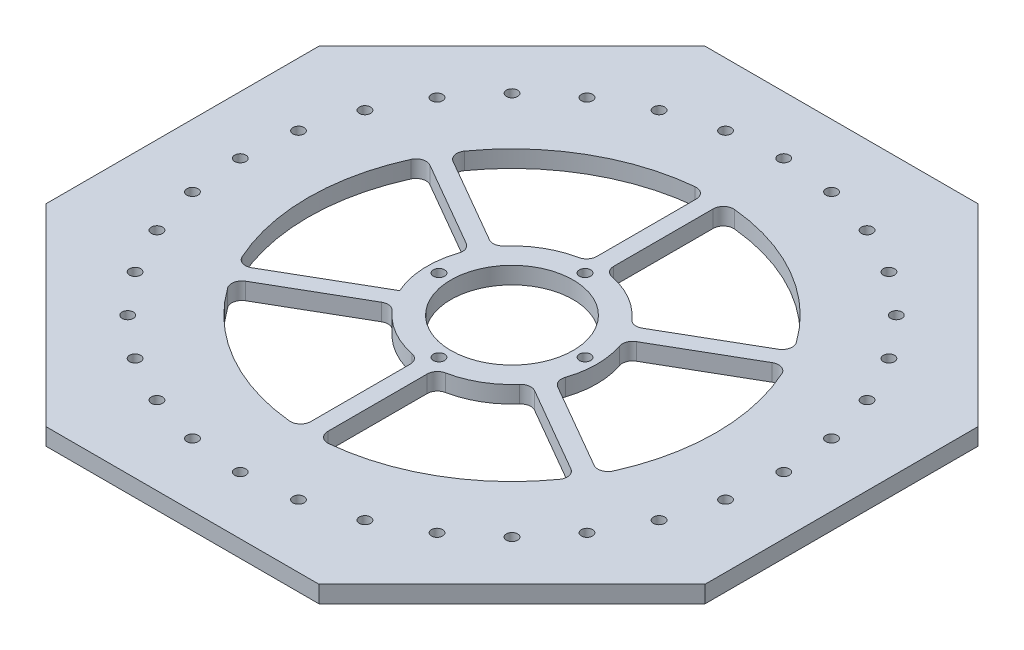
from build123d import *

# Parameters (mm, degrees)
SKETCH_1_R               = 25
SKETCH_1_R_2             = 18
EXTRUDE_1_DEPTH          = 2.5
SKETCH_1_R_3             = 60
EXTRUDE_1_2_DEPTH        = 2.5
SKETCH_8_W               = 5
SKETCH_8_H               = 39.844025058
EXTRUDE_2_DEPTH          = 5
PATTERN_CIRCULAR_3_COUNT = 6
EXTRUDE_START            = 12
SKETCH_9_R               = 25
SKETCH_9_R_2             = 18
EXTRUDE_3_DEPTH          = 12
SKETCH_11_R              = 1.65
CUT_EXTRUDE_3_DEPTH      = 8
PATTERN_CIRCULAR_5_COUNT = 32
SKETCH_12_R              = 2.2
CUT_EXTRUDE_4_DEPTH      = 45
CUT_EXTRUDE_START        = -24
SKETCH_13_R              = 4
CUT_EXTRUDE_5_DEPTH      = 45
PATTERN_CIRCULAR_6_COUNT = 4
SKETCH_14_R              = 25
CUT_EXTRUDE_6_DEPTH      = 12
FILLET_1_R               = 3
SKETCH_15_R              = 1.65
CUT_EXTRUDE_7_DEPTH      = 10
PATTERN_CIRCULAR_7_COUNT = 4


with BuildPart() as part:
    # 草图1 → 凸台-拉伸1 (new, symmetric)
    with BuildSketch(Plane(origin=(0, 0, 0), x_dir=(1, 0, 0), z_dir=(0, 1, 0))):
        with Locations(Location((0, 0, 0), (0, 0, 270))):
            Circle(SKETCH_1_R)
        with Locations(Location((0, 0, 0), (0, 0, 270))):
            Circle(SKETCH_1_R_2, mode=Mode.SUBTRACT)
    extrude(amount=EXTRUDE_1_DEPTH, both=True)



with BuildPart() as body_2:
    # 草图1 → Extrude 1 2 (new, symmetric)
    with BuildSketch(Plane(origin=(0, 0, 0), x_dir=(1, 0, 0), z_dir=(0, 1, 0))):
        Polygon((97.007350914, 40.181760398), (40.181760398, 97.007350914), (-40.181760398, 97.007350914), (-97.007350914, 40.181760398), (-97.007350914, -40.181760398), (-40.181760398, -97.007350914), (40.181760398, -97.007350914), (97.007350914, -40.181760398), align=None)
        with Locations(Location((0, 0, 0), (0, 0, 270))):
            Circle(SKETCH_1_R_3, mode=Mode.SUBTRACT)
    extrude(amount=EXTRUDE_1_2_DEPTH, both=True)


with BuildPart() as part_1:
    add(part.part)

    add(body_2.part)  # 凸台-拉伸2 merges body 2
    # 草图8 → 凸台-拉伸2 (add)
    with BuildSketch(Plane(origin=(0, 2.5, 0), x_dir=(1, 0, 0), z_dir=(0, 1, 0))):
        with Locations((0, 44.796698457)):
            Rectangle(SKETCH_8_W, SKETCH_8_H)
    extrude_2 = extrude(amount=-EXTRUDE_2_DEPTH)

    # 阵列(圆周)3: 凸台-拉伸2 ×6 about axis
    pattern_circular_3_axis = Axis((0, 0, 0), (0, 1, 0))
    for i in range(1, PATTERN_CIRCULAR_3_COUNT):
        add(extrude_2.rotate(pattern_circular_3_axis, i * 360 / PATTERN_CIRCULAR_3_COUNT))

    # 草图9 → 凸台-拉伸3 (add)
    with BuildSketch(Plane(origin=(0, 2.5, 0), x_dir=(1, 0, 0), z_dir=(0, 1, 0)).offset(EXTRUDE_START)):
        with Locations(Location((0, 0, 0), (0, 0, 84.260829523))):
            Circle(SKETCH_9_R)
        with Locations(Location((0, 0, 0), (0, 0, 270))):
            Circle(SKETCH_9_R_2, mode=Mode.SUBTRACT)
    extrude(amount=-EXTRUDE_3_DEPTH)

    # 草图11 → 切除-拉伸3 (cut)
    with BuildSketch(Plane(origin=(0, 2.5, 0), x_dir=(1, 0, 0), z_dir=(0, 1, 0))):
        with Locations(Location((0, 80, 0), (0, 0, 270))):
            Circle(SKETCH_11_R)
    cut_extrude_3 = extrude(amount=-CUT_EXTRUDE_3_DEPTH, mode=Mode.SUBTRACT)

    # 阵列(圆周)5: 切除-拉伸3 ×32 about axis
    pattern_circular_5_axis = Axis((0, 0, 0), (0, 1, 0))
    for i in range(1, PATTERN_CIRCULAR_5_COUNT):
        add(cut_extrude_3.rotate(pattern_circular_5_axis, i * 360 / PATTERN_CIRCULAR_5_COUNT), mode=Mode.SUBTRACT)

    # 草图12 → 切除-拉伸4 (cut)
    with BuildSketch(Plane.XY):
        with Locations(Location((0, 9.5, 0), (0, 0, 90))):
            Circle(SKETCH_12_R)
    cut_extrude_4 = extrude(amount=-CUT_EXTRUDE_4_DEPTH, mode=Mode.SUBTRACT)

    # 草图13 → 切除-拉伸5 (cut)
    with BuildSketch(Plane.XY.offset(CUT_EXTRUDE_START)):
        with Locations((0, 9.5)):
            Circle(SKETCH_13_R)
    cut_extrude_5 = extrude(amount=-CUT_EXTRUDE_5_DEPTH, mode=Mode.SUBTRACT)

    # 阵列(圆周)6: 切除-拉伸4, 切除-拉伸5 ×4 about axis
    pattern_circular_6_axis = Axis((0, 0, 0), (0, 1, 0))
    add([cut_extrude_4.rotate(pattern_circular_6_axis, i * 360 / PATTERN_CIRCULAR_6_COUNT) for i in range(1, PATTERN_CIRCULAR_6_COUNT)], mode=Mode.SUBTRACT)
    add([cut_extrude_5.rotate(pattern_circular_6_axis, i * 360 / PATTERN_CIRCULAR_6_COUNT) for i in range(1, PATTERN_CIRCULAR_6_COUNT)], mode=Mode.SUBTRACT)

    # 草图14 → 切除-拉伸6 (cut)
    with BuildSketch(Plane(origin=(0, 14.5, 0), x_dir=(1, 0, 0), z_dir=(0, 1, 0))):
        Circle(SKETCH_14_R)
    extrude(amount=-CUT_EXTRUDE_6_DEPTH, mode=Mode.SUBTRACT)

    # 圆角1
    fillet_1_edges = [part_1.edges().sort_by_distance(p)[0] for p in [
        (2.5, 0, 59.947894041),
        (2.5, 0, 24.874685928),
        (-2.5, 0, 59.947894041),
        (-2.5, 0, 24.874685928),
        (-50.666399143, 0, 32.13901053),
        (-20.292109925, 0, 14.602406473),
        (-53.166399143, 0, 27.808883511),
        (-53.166399143, 0, -27.808883511),
        (-22.792109925, 0, -10.272279454),
        (-50.666399143, 0, -32.13901053),
        (-20.292109925, 0, -14.602406473),
        (-2.5, 0, -59.947894041),
        (-2.5, 0, -24.874685928),
        (2.5, 0, -59.947894041),
        (2.5, 0, -24.874685928),
        (50.666399143, 0, -32.13901053),
        (20.292109925, 0, -14.602406473),
        (53.166399143, 0, -27.808883511),
        (22.792109925, 0, -10.272279454),
        (53.166399143, 0, 27.808883511),
        (22.792109925, 0, 10.272279454),
        (50.666399143, 0, 32.13901053),
        (20.292109925, 0, 14.602406473),
    ]]
    fillet(fillet_1_edges, radius=FILLET_1_R)

    # 草图15 → 切除-拉伸7 (cut)
    with BuildSketch(Plane(origin=(0, 2.5, 0), x_dir=(1, 0, 0), z_dir=(0, 1, 0))):
        with Locations(Location((0, 21.5, 0), (0, 0, 270))):
            Circle(SKETCH_15_R)
    cut_extrude_7 = extrude(amount=-CUT_EXTRUDE_7_DEPTH, mode=Mode.SUBTRACT)

    # 阵列(圆周)7: 切除-拉伸7 ×4 about axis
    pattern_circular_7_axis = Axis((0, 0, 0), (0, 1, 0))
    for i in range(1, PATTERN_CIRCULAR_7_COUNT):
        add(cut_extrude_7.rotate(pattern_circular_7_axis, i * 360 / PATTERN_CIRCULAR_7_COUNT), mode=Mode.SUBTRACT)


solid = part_1.part
